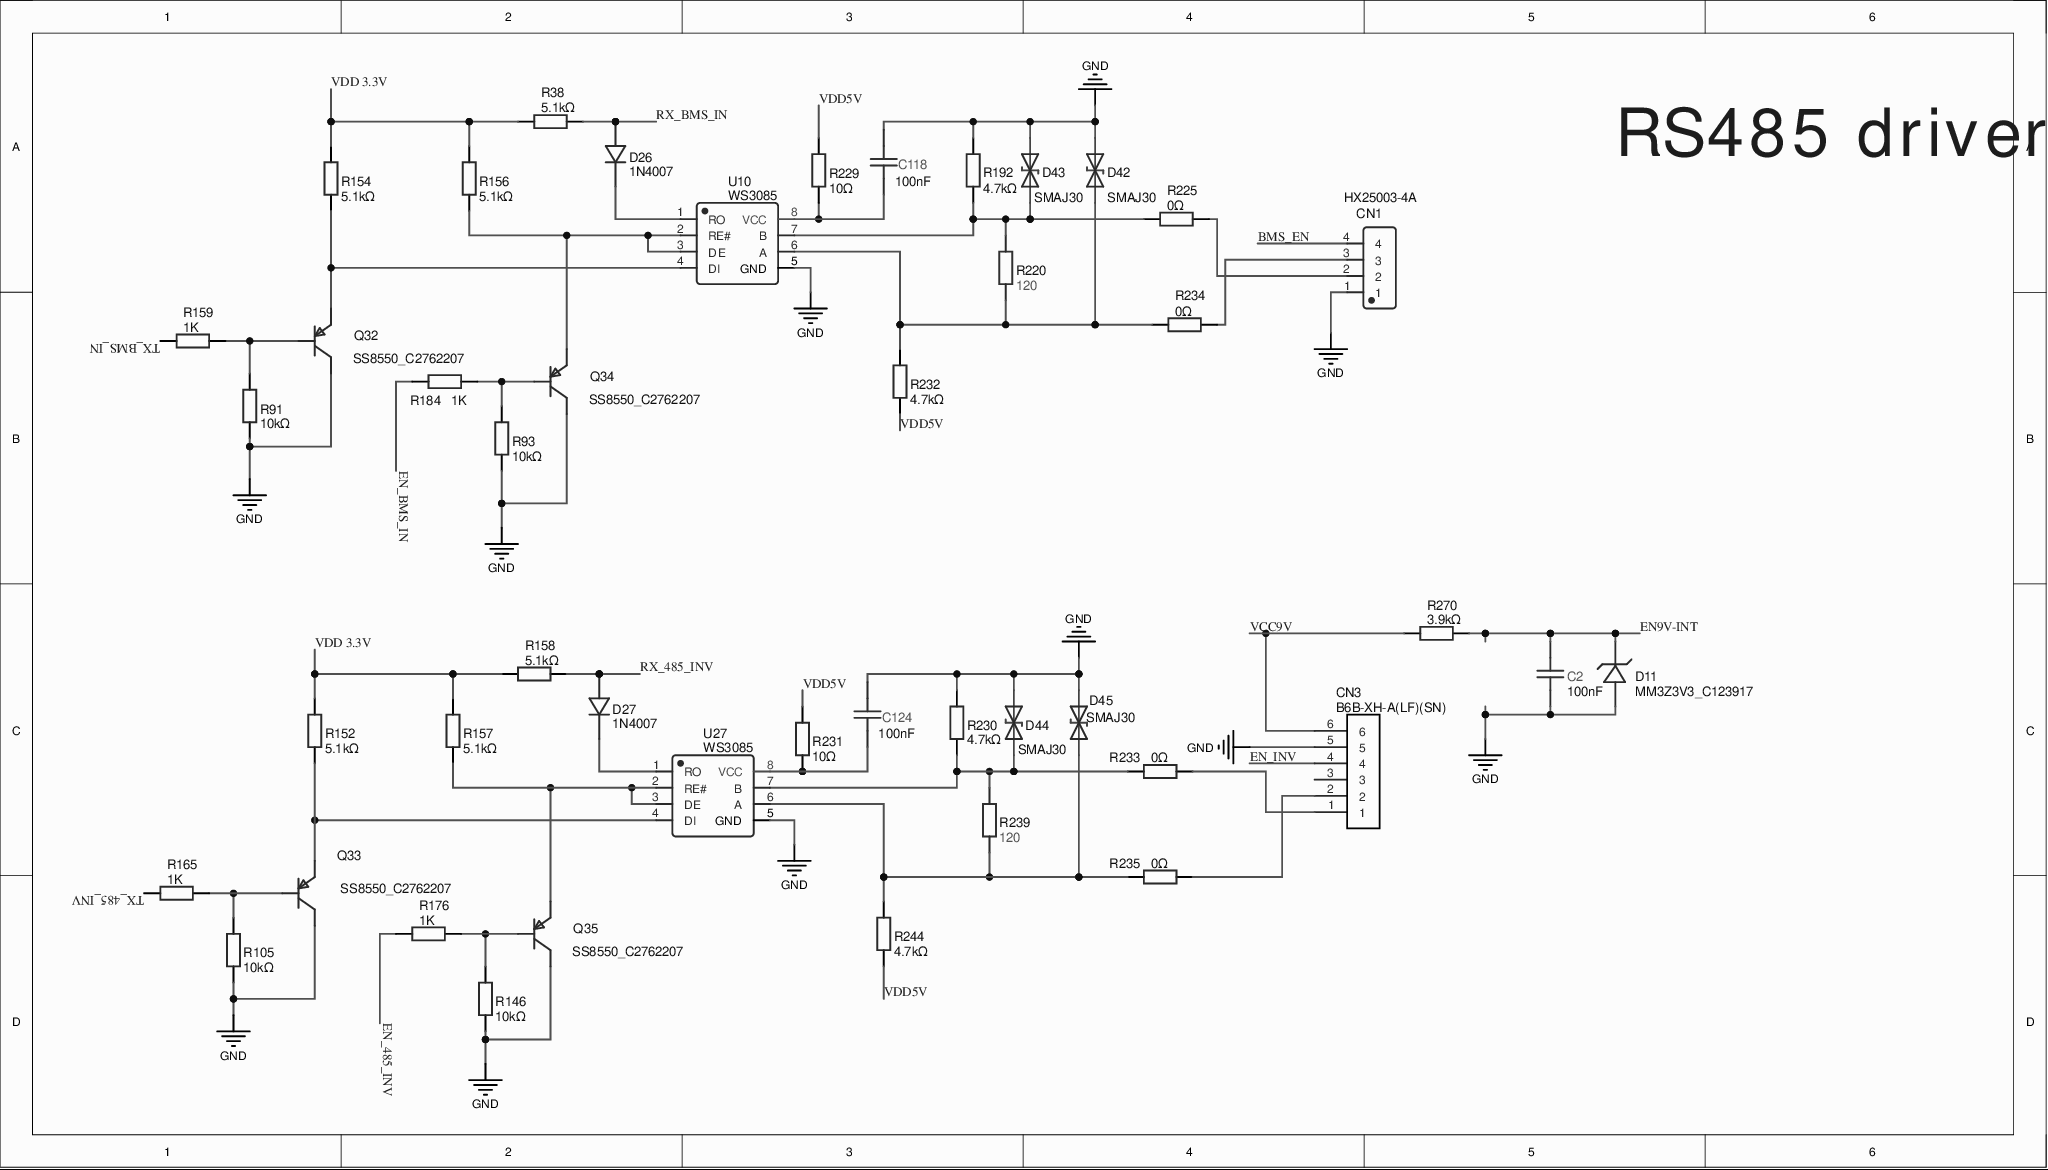
[diagram p0: MISC84402-10.SchDoc]
# Altium project MISC84402-4.PrjPcb (part 3 of 7)

## Sheet MISC84402-10.SchDoc
size 319 x 182 mm

### Parts
C2  100nF  [C0603]
C118  100nF  [C0603]
C124  100nF  [C0603]
CN1  HX25003-4A  [CONN-TH_4P-P2.50_HX25003-4A]
CN3  B6B-XH-A(LF)(SN)  [CONN-TH_6P-P2.50_B6B-XH-A-LF-SN]
D11  MM3Z3V3_C123917  [SOD-323_L1.8-W1.3-LS2.5-RD]
D26  1N4007  [DO-41_BD2.4-L4.7-P8.70-D0.9-RD]
D27  1N4007  [DO-41_BD2.4-L4.7-P8.70-D0.9-RD]
D42  SMAJ30  [SMA_L4.3-W2.5-LS5.0-BI]
D43  SMAJ30  [SMA_L4.3-W2.5-LS5.0-BI]
D44  SMAJ30  [SMA_L4.3-W2.5-LS5.0-BI]
D45  SMAJ30  [SMA_L4.3-W2.5-LS5.0-BI]
Q32  SS8550_C2762207  [SOT-23-3_L2.9-W1.3-P1.90-LS2.4-BR]
Q33  SS8550_C2762207  [SOT-23-3_L2.9-W1.3-P1.90-LS2.4-BR]
Q34  SS8550_C2762207  [SOT-23-3_L2.9-W1.3-P1.90-LS2.4-BR]
Q35  SS8550_C2762207  [SOT-23-3_L2.9-W1.3-P1.90-LS2.4-BR]
R38  5.1kΩ  [R0603]
R91  10kΩ  [R0603]
R93  10kΩ  [R0603]
R105  10kΩ  [R0603]
R146  10kΩ  [R0603]
R152  5.1kΩ  [R0603]
R154  5.1kΩ  [R0603]
R156  5.1kΩ  [R0603]
R157  5.1kΩ  [R0603]
R158  5.1kΩ  [R0603]
R159  1K  [R0603]
R165  1K  [R0603]
R176  1K  [R0603]
R184  1K  [R0603]
R192  4.7kΩ  [R0603]
R220  120  [R1206]
R225  0Ω  [R0603]
R229  10Ω  [R0603]
R230  4.7kΩ  [R0603]
R231  10Ω  [R0603]
R232  4.7kΩ  [R0603]
R233  0Ω  [R0603]
R234  0Ω  [R0603]
R235  0Ω  [R0603]
R239  120  [R1206]
R244  4.7kΩ  [R0603]
R270  3.9kΩ  [R0603]
U10  WS3085  [SOP-8_L5.0-W4.0-P1.27-LS6.0-BL]
U27  WS3085  [SOP-8_L5.0-W4.0-P1.27-LS6.0-BL]

### Nets
GND: C2.1 C118.2 C124.2 CN1.1 CN3.5 D11.2(A) D42.2 D43.2 D44.2 D45.2 Q32.3(C) Q33.3(C) Q34.3(C) Q35.3(C) R91.1 R93.1 R105.1 R146.1 R192.2 R230.2 U10.5(GND) U27.5(GND)
BMS_EN: CN1.4
EN9V-INT: C2.2 D11.1(K) R270.2
EN_485_INV: R176.1
EN_BMS_IN: R184.1
EN_INV: CN3.4
RX_485_INV: D27.2 R158.2
RX_BMS_IN: D26.2 R38.2
TX_485_INV: R165.1
TX_BMS_IN: R159.1
VCC9V: CN3.6 R270.1
VDD5V: R229.2 R231.2 R232.1 R244.1
VDD 3.3V: R38.1 R152.2 R154.2 R156.2 R157.2 R158.1
NetC118_1: C118.1 R229.1 U10.8(VCC)
NetC124_1: C124.1 R231.1 U27.8(VCC)
NetCN1_2: CN1.2 R225.2
NetCN1_3: CN1.3 R234.2
NetCN3_1: CN3.1 R233.2
NetCN3_2: CN3.2 R235.2
NetD26_1: D26.1 U10.1(RO)
NetD27_1: D27.1 U27.1(RO)
NetD42_1: D42.1 R220.1 R232.2 R234.1 U10.6(A)
NetD43_1: D43.1 R192.1 R220.2 R225.1 U10.7(B)
NetD44_1: D44.1 R230.1 R233.1 R239.1 U27.7(B)
NetD45_1: D45.1 R235.1 R239.2 R244.2 U27.6(A)
NetQ32_1: Q32.1(B) R91.2 R159.2
NetQ32_2: Q32.2(E) R154.1 U10.4(DI)
NetQ33_1: Q33.1(B) R105.2 R165.2
NetQ33_2: Q33.2(E) R152.1 U27.4(DI)
NetQ34_1: Q34.1(B) R93.2 R184.2
NetQ34_2: Q34.2(E) R156.1 U10.2(RE#) U10.3(DE)
NetQ35_1: Q35.1(B) R146.2 R176.2
NetQ35_2: Q35.2(E) R157.1 U27.2(RE#) U27.3(DE)

Not connected (* = marked no-connect by the designer): CN3 3

### Notes on the sheet
- RS485 driver circuit

### Library data of the parts
C2 C118 C124 = 100nF: BOM_Manufacturer: SAMSUNG; BOM_Manufacturer Part: CL10B104KC8NNNC; nameAlias: Capacitance; BOM_Supplier: LCSC; BOM_Supplier Part: C15725; BOM_JLCPCB Part Class: Extended Part; spicePre: C; spiceSymbolName: CL10B104KC8NNNC
CN1 = HX25003-4A: BOM_Manufacturer: HX(Zhejiang Yueqing Hongxing Elec); Contributor: LCSC; BOM_Supplier: LCSC; BOM_Supplier Part: C442301; BOM_Manufacturer Part: HX25003-4A; BOM_JLCPCB Part Class: Extended Part; spicePre: C; spiceSymbolName: HX25003-4A
CN3 = B6B-XH-A(LF)(SN): BOM_Manufacturer: JST Sales America; Contributor: LCSC; BOM_Supplier: LCSC; BOM_Supplier Part: C144397; BOM_Manufacturer Part: B6B-XH-A(LF)(SN); BOM_JLCPCB Part Class: Extended Part; spicePre: U; spiceSymbolName: B6B-XH-A(LF)(SN)
D11 = MM3Z3V3_C123917: BOM_Manufacturer: Shandong Jingdao Microelectronics; Contributor: LCSC; BOM_Supplier: LCSC; BOM_Supplier Part: C123917; BOM_Manufacturer Part: MM3Z3V3; BOM_JLCPCB Part Class: Extended Part; spicePre: D; spiceSymbolName: MM3Z3V3_C123917
D26 D27 = 1N4007: BOM_Manufacturer: SEMTECH; Contributor: LCEDA_Lib; BOM_Supplier: LCSC; BOM_Manufacturer Part: 1N4007; BOM_Supplier Part: C106903; spicePre: D; spiceSymbolName: 1N4007
D42-D45 = SMAJ30: BOM_Manufacturer: Shandong Jingdao Microelectronics; BOM_Manufacturer Part: SMAJ30CA; Contributor: LCSC; BOM_Supplier: LCSC; BOM_Supplier Part: C353455; BOM_JLCPCB Part Class: Extended Part; spicePre: D; spiceSymbolName: SMAJ30CA_C353455
Q32-Q35 = SS8550_C2762207: BOM_Manufacturer: Jingdao Microelectronics; BOM_Manufacturer Part: SS8550; Contributor: LCSC; BOM_Supplier: LCSC; BOM_Supplier Part: C2762207; BOM_JLCPCB Part Class: Extended Part; spicePre: Q; spiceSymbolName: SS8550_C2762207
R38 R152 R154 R156-R158 = 5.1kΩ: BOM_Manufacturer Part: 0603WAF5101T5E; BOM_Manufacturer: UniOhm; Resistance (Ohms): 5.1K; nameAlias: Resistance; BOM_Supplier: LCSC; BOM_Supplier Part: C23186; BOM_JLCPCB Part Class: Basic Part; spicePre: R; spiceSymbolName: 0603WAF5101T5E
R91 R93 R105 R146 = 10kΩ: BOM_Manufacturer: UniOhm; BOM_Manufacturer Part: 0603WAF1002T5E; nameAlias: Resistance; Resistance (Ohms): 10K; BOM_Supplier: LCSC; BOM_Supplier Part: C25804; BOM_JLCPCB Part Class: Basic Part; spicePre: R; spiceSymbolName: 0603WAF1002T5E
R159 R165 R176 R184 = 1K: BOM_Manufacturer: FH; BOM_Manufacturer Part: RS-03K102JT; nameAlias: Resistance (Ohms); BOM_Supplier: LCSC; BOM_Supplier Part: C73797; spicePre: R; spiceSymbolName: RS-03K102JT
R192 R230 R232 R244 = 4.7kΩ: BOM_Manufacturer: UniOhm; BOM_Manufacturer Part: 0603WAF4701T5E; nameAlias: Resistance; Resistance (Ohms): 4.7K; BOM_Supplier: LCSC; BOM_Supplier Part: C23162; BOM_JLCPCB Part Class: Basic Part; spicePre: R; spiceSymbolName: 0603WAF4701T5E
R220 R239 = 120: BOM_Manufacturer: Viking Tech; BOM_Manufacturer Part: ARG06FTC1200; nameAlias: Resistance (Ohms); Contributor: LCSC; BOM_Supplier: LCSC; BOM_Supplier Part: C294122; BOM_JLCPCB Part Class: Extended Part; spicePre: R; spiceSymbolName: ARG06FTC1200
R225 R233-R235 = 0Ω: BOM_Manufacturer: UniOhm; BOM_Manufacturer Part: 0603WAF0000T5E; nameAlias: Resistance; Resistance (Ohms): 0; BOM_Supplier: LCSC; BOM_Supplier Part: C21189; BOM_JLCPCB Part Class: Basic Part; spicePre: R; spiceSymbolName: 0603WAF0000T5E
R229 R231 = 10Ω: BOM_Manufacturer: UniOhm; BOM_Manufacturer Part: 0603WAF100JT5E; nameAlias: Resistance; BOM_Supplier: LCSC; BOM_Supplier Part: C22859; Resistance (Ohms): 10Ω; BOM_JLCPCB Part Class: Basic Part; spicePre: R; spiceSymbolName: 0603WAF100JT5E
R270 = 3.9kΩ: BOM_Manufacturer: UniOhm; BOM_Manufacturer Part: 0603WAF3901T5E; nameAlias: Resistance; Resistance (Ohms): 3.9K; BOM_Supplier: LCSC; BOM_Supplier Part: C23018; BOM_JLCPCB Part Class: Basic Part; spicePre: R; spiceSymbolName: 0603WAF3901T5E
U10 U27 = WS3085: BOM_Manufacturer: GEC (Nanjing Guobo); Contributor: LCSC; BOM_Supplier: LCSC; BOM_Supplier Part: C2691412; BOM_Manufacturer Part: WS3085; BOM_JLCPCB Part Class: Extended Part; spicePre: U; spiceSymbolName: WS3085

## Sheet MISC84402-9.SchDoc
size 225 x 98 mm
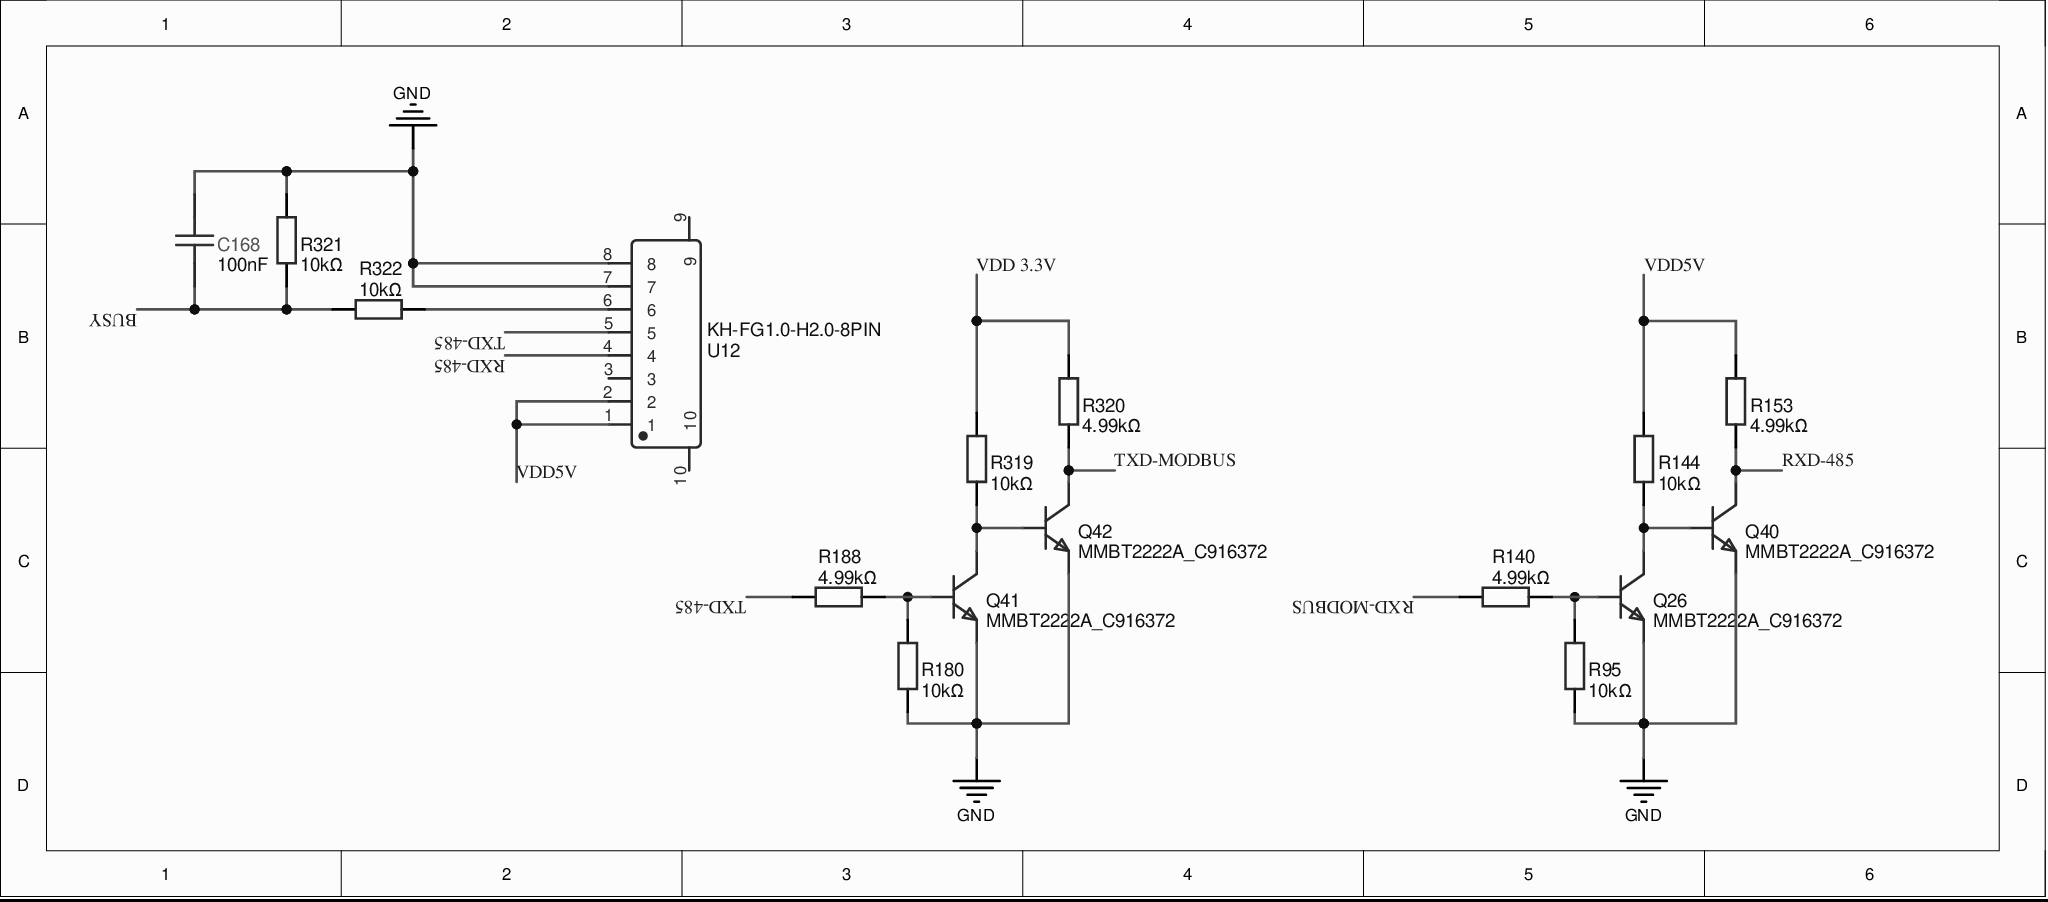
[diagram p1: MISC84402-9.SchDoc]

### Parts
C168  100nF  [C0603]
Q26  MMBT2222A_C916372  [SOT-23-3_L2.9-W1.3-P1.90-LS2.4-BR]
Q40  MMBT2222A_C916372  [SOT-23-3_L2.9-W1.3-P1.90-LS2.4-BR]
Q41  MMBT2222A_C916372  [SOT-23-3_L2.9-W1.3-P1.90-LS2.4-BR]
Q42  MMBT2222A_C916372  [SOT-23-3_L2.9-W1.3-P1.90-LS2.4-BR]
R95  10kΩ  [R0603]
R140  4.99kΩ  [R0603]
R144  10kΩ  [R0603]
R153  4.99kΩ  [R0603]
R180  10kΩ  [R0603]
R188  4.99kΩ  [R0603]
R319  10kΩ  [R0603]
R320  4.99kΩ  [R0603]
R321  10kΩ  [R0603]
R322  10kΩ  [R0603]
U12  KH-FG1.0-H2.0-8PIN  [FPC-SMD_KH-FG1.0-H2.0-8PIN]

### Nets
GND: C168.1 Q26.2(E) Q40.2(E) Q41.2(E) Q42.2(E) R95.1 R180.1 R321.2 U12.7 U12.8
BUSY: C168.2 R321.1 R322.2
RXD-485: Q40.3(C) R153.1 U12.4
RXD-MODBUS: R140.1
TXD-485: R188.2 U12.5
TXD-MODBUS: Q42.3(C) R320.1
VDD5V: R144.2 R153.2 U12.1 U12.2
VDD 3.3V: R319.2 R320.2
NetQ26_1: Q26.1(B) R95.2 R140.2
NetQ26_3: Q26.3(C) Q40.1(B) R144.1
NetQ41_1: Q41.1(B) R180.2 R188.1
NetQ41_3: Q41.3(C) Q42.1(B) R319.1
NetR322_1: R322.1 U12.6

Not connected (* = marked no-connect by the designer): U12 3 9 10

### Library data of the parts
C168 = 100nF: as C2 on sheet MISC84402-10; BOM_Supplier: LCSC; BOM_Supplier Part: C15725; BOM_JLCPCB Part Class: Extended Part; spicePre: C; spiceSymbolName: CL10B104KC8NNNC
Q26 Q40-Q42 = MMBT2222A_C916372: BOM_Manufacturer: JSMSEMI; Contributor: LCSC; BOM_Supplier: LCSC; BOM_Supplier Part: C916372; BOM_Manufacturer Part: MMBT2222A; BOM_JLCPCB Part Class: Extended Part; spicePre: Q; spiceSymbolName: MMBT2222A_C916372
R95 R144 R180 R319 R321 R322 = 10kΩ: as R91 on sheet MISC84402-10; BOM_Supplier: LCSC; BOM_Supplier Part: C25804; BOM_JLCPCB Part Class: Basic Part; spicePre: R; spiceSymbolName: 0603WAF1002T5E
R140 R153 R188 R320 = 4.99kΩ: BOM_Manufacturer: UniOhm; BOM_Manufacturer Part: 0603WAF4991T5E; nameAlias: Resistance; Resistance (Ohms): 4.99K; BOM_Supplier: LCSC; BOM_Supplier Part: C23046; BOM_JLCPCB Part Class: Basic Part; spicePre: R; spiceSymbolName: 0603WAF4991T5E
U12 = KH-FG1.0-H2.0-8PIN: BOM_Manufacturer: Kinghelm; Contributor: LCSC; BOM_Supplier: LCSC; BOM_Supplier Part: C2797225; BOM_Manufacturer Part: KH-FG1.0-H2.0-8PIN; BOM_JLCPCB Part Class: Extended Part; spicePre: C; spiceSymbolName: KH-FG1.0-H2.0-8PIN

## Sheet MISC84402-11.SchDoc
size 345 x 185 mm
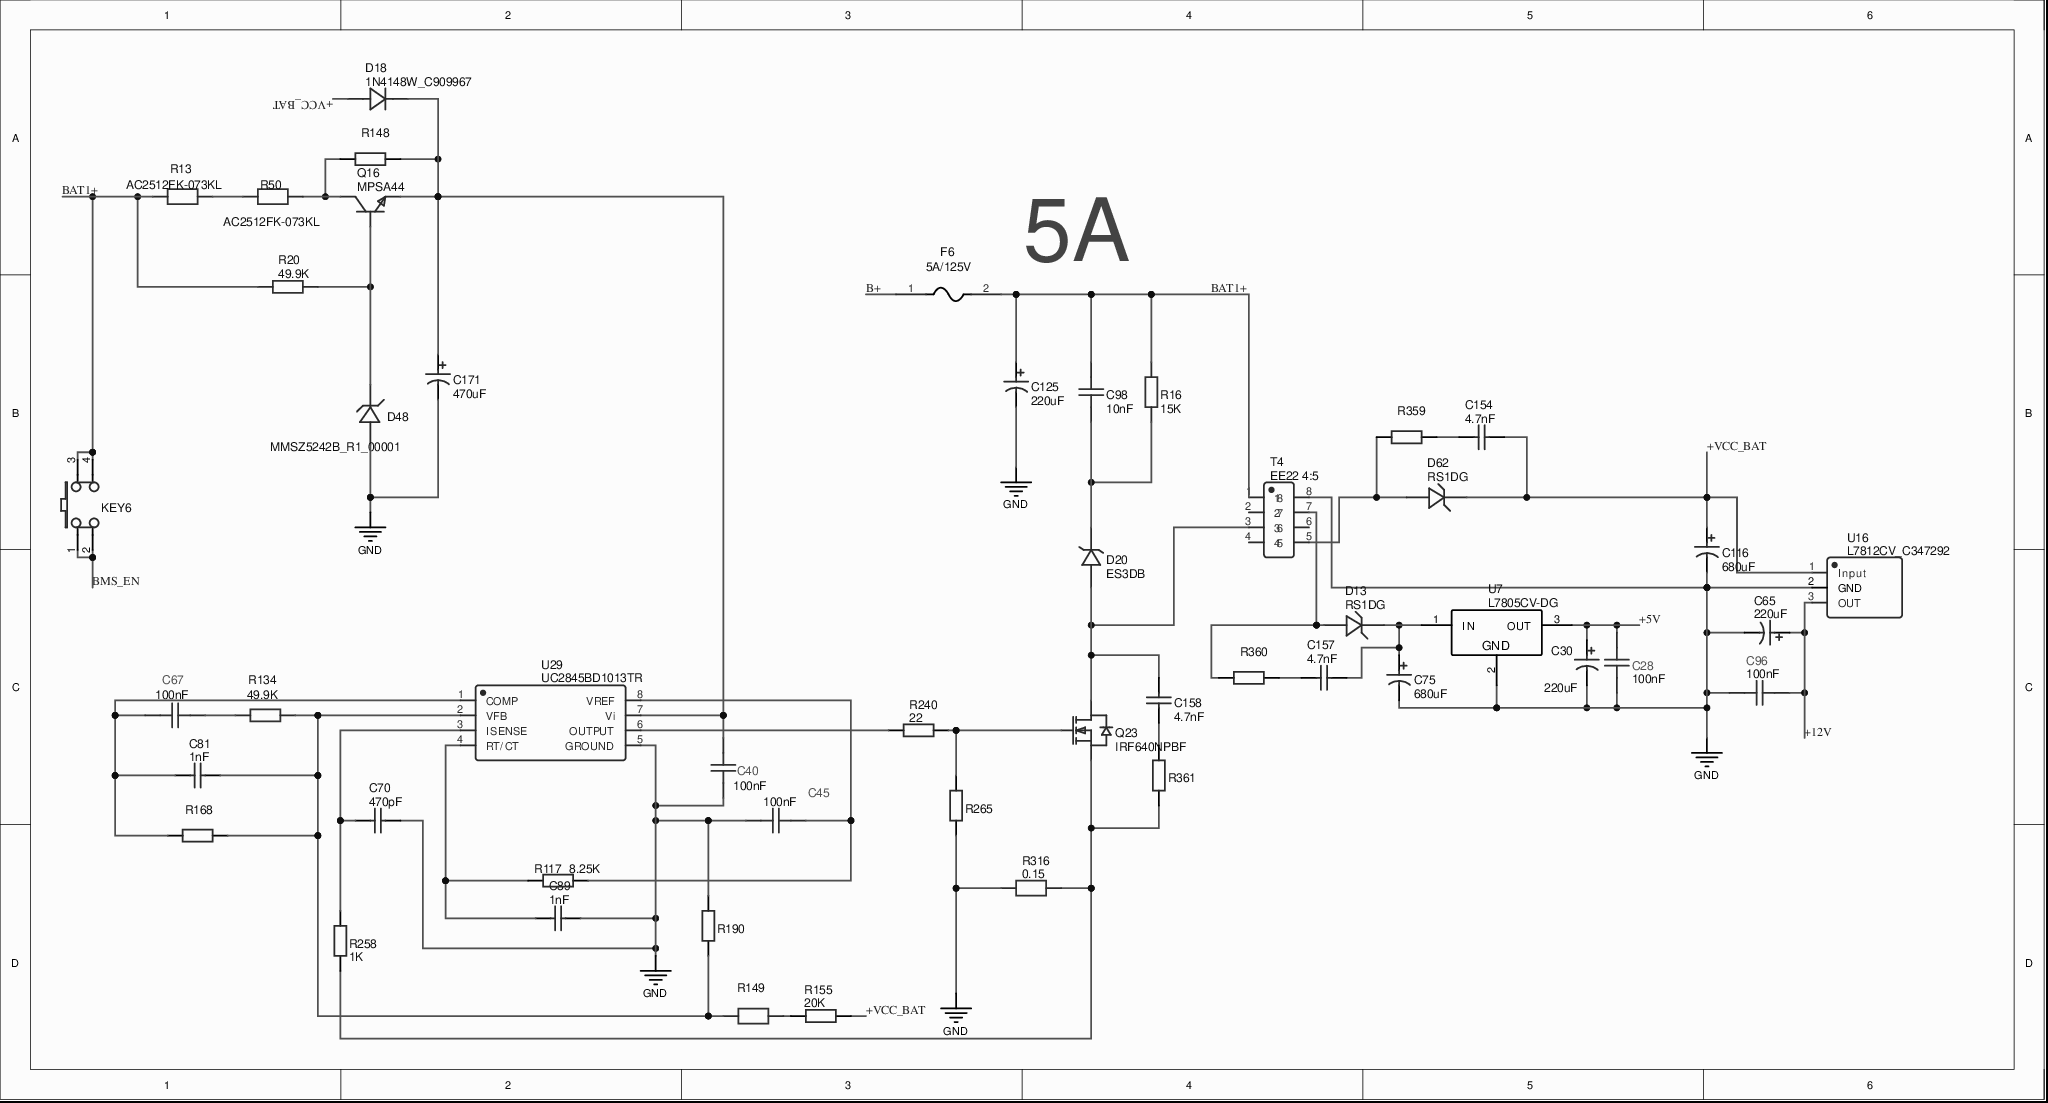
[diagram p2: MISC84402-11.SchDoc]

### Parts
C28  100nF  [C0603]
C30  220uF  [CAP-TH_BD6.3-P2.50-D1.0-FD]
C40  100nF  [C0603]
C45  100nF  [C0603]
C65  220uF  [CAP-TH_BD6.3-P2.50-D1.0-FD]
C67  100nF  [C0603]
C70  470pF  [C0603]
C75  680uF  [CAP-TH_BD10.0-P5.00-D1.0-FD]
C81  1nF  [C0603]
C89  1nF  [C0603]
C96  100nF  [C0603]
C98  10nF  [CAP-TH_L8.0-W4.0-P5.00-D1.2]
C116  680uF  [CAP-TH_BD10.0-P5.00-D1.0-FD]
C125  220uF  [CAP-TH_BD10.0-P5.00-D1.0-FD]
C154  4.7nF  [C1206]
C157  4.7nF  [C1206]
C158  4.7nF  [C1206]
C171  470uF  [CAP-TH_BD12.5-P5.00-D0.6-FD]
D13  RS1DG  [SMA_L4.4-W2.8-LS5.4-RD]
D18  1N4148W_C909967  [SOD-123_L2.8-W1.8-LS3.7-RD]
D20  ES3DB  [SMB_L4.6-W3.6-LS5.3-RD]
D48  MMSZ5242B_R1_00001  [SOD-123_L2.7-W1.6-LS3.7-RD-1]
D62  RS1DG  [SMA_L4.4-W2.8-LS5.4-RD]
F6  5A/125V  [FUSE-SMD_L6.1-W2.5]
KEY6  4-1437565-2  [SW-SMD_4P-L6.0-W6.0-P4.50-LS8.6]  (value not drawn)
Q16  MPSA44  [TO-92-3_L4.8-W3.7-P2.54-L]
Q23  IRF640NPBF  [TO-220-3_L10.0-W4.5-P2.54-L]
R13  AC2512FK-073KL  [R2512]
R16  15K  [RES-TH_BD3.3-L9.0-P13.00-D0.6]
R20  49.9K  [R0603]
R50  AC2512FK-073KL  [R2512]
R117  8.25K  [R0603]
R134  49.9K  [R0603]
R148  (no value)  [R0603]
R149  (no value)  [R0603]
R155  20K  [R0603]
R168  (no value)  [R0603]
R190  (no value)  [R0603]
R240  22  [R0603]
R258  1K  [R0603]
R265  (no value)  [R0603]
R316  0.15  [R2512]
R359  (no value)  [R1206]
R360  (no value)  [R1206]
R361  (no value)  [R1206]
T4  EE22 4:5  [EE22 4:5NEW]
U7  L7805CV-DG  [TO-220-3_L10.0-W4.5-P2.54-L]
U16  L7812CV_C347292  [TO-220-3_L10.0-W4.5-P2.54-L]
U29  UC2845BD1013TR  [SOP-8_L4.9-W3.9-P1.27-LS6.0-BL]

### Nets
GND: C28.2 C30.2 C40.1 C45.2 C65.2 C70.2 C75.2 C89.2 C96.2 C116.2 C125.2 C171.2 D48.2(A) R190.2 R265.1 R316.1 T4.8 U7.2(GND) U16.2(GND) U29.5(GROUND)
+5V: C28.1 C30.1 U7.3(OUT)
+12V: C65.1 C96.1 U16.3(OUT)
+VCC_BAT: C116.1 C154.1 D18.2(A) D62.1(C) R155.1 U16.1(Input)
B+: F6.1
BAT1+: C98.2 C125.1 F6.2 KEY6.3 KEY6.4 R13.2 R16.2 R20.1 T4.1
BMS_EN: KEY6.1 KEY6.2
NetC40_2: C40.2 C171.1 D18.1(K) Q16.1(E) R148.2 U29.7(Vi)
NetC45_1: C45.1 R117.2 U29.8(VREF)
NetC67_1: C67.1 R134.1
NetC67_2: C67.2 C81.1 R168.2 U29.1(COMP)
NetC70_1: C70.1 R258.2 U29.3(ISENSE)
NetC75_1: C75.1 C157.1 D13.1(C) U7.1(IN)
NetC81_2: C81.2 R134.2 R149.2 R168.1 R190.1 U29.2(VFB)
NetC89_1: C89.1 R117.1 U29.4(RT/CT)
NetC98_1: C98.1 D20.1(C) R16.1
NetC154_2: C154.2 R359.2
NetC157_2: C157.2 R360.2
NetC158_1: C158.1 R361.2
NetC158_2: C158.2 D20.2(A) Q23.2(D) T4.3
NetD13_2: D13.2(A) R360.1 T4.7
NetD48_1: D48.1(K) Q16.2(B) R20.2
NetD62_2: D62.2(A) R359.1 T4.5
NetQ16_3: Q16.3(C) R50.1 R148.1
NetQ23_1: Q23.1(G) R240.2 R265.2
NetQ23_3: Q23.3(S) R258.1 R316.2 R361.1
NetR13_1: R13.1 R50.2
NetR149_1: R149.1 R155.2
NetR240_1: R240.1 U29.6(OUTPUT)

Not connected (* = marked no-connect by the designer): T4 2 4 6

### Notes on the sheet
- (near F6) 5A

### Library data of the parts
C28 C40 C45 C67 C96 = 100nF: as C2 on sheet MISC84402-10; BOM_Supplier: LCSC; BOM_Supplier Part: C15725; BOM_JLCPCB Part Class: Extended Part; spicePre: C; spiceSymbolName: CL10B104KC8NNNC
C30 C65 = 220uF: BOM_Manufacturer: ValuePro; BOM_Manufacturer Part: 220uF 16V 6.3*11; nameAlias: Capacitance; BOM_Supplier: LCSC; BOM_Supplier Part: C43349; BOM_JLCPCB Part Class: Extended Part; spicePre: C; spiceSymbolName: 220uF 16V 6.3*11
C70 = 470pF: BOM_Manufacturer: FH; BOM_Manufacturer Part: 0603B471K500NT; nameAlias: Capacitance; BOM_Supplier: LCSC; BOM_Supplier Part: C1620; BOM_JLCPCB Part Class: Basic Part; spicePre: C; spiceSymbolName: 0603B471K500NT
C75 C116 = 680uF: BOM_Manufacturer: ValuePro; BOM_Manufacturer Part: high frequency 680uF35V; nameAlias: Capacitance; BOM_Supplier: LCSC; BOM_Supplier Part: C23777; BOM_JLCPCB Part Class: Extended Part; spicePre: C; spiceSymbolName: high frequency 680uF35V
C81 C89 = 1nF: BOM_Manufacturer Part: CL10B102KB8NNNC; BOM_Manufacturer: SAMSUNG; nameAlias: Capacitance; BOM_Supplier: LCSC; BOM_Supplier Part: C1588; BOM_JLCPCB Part Class: Basic Part; spicePre: C; spiceSymbolName: CL10B102KB8NNNC
C98 = 10nF: BOM_Manufacturer: Songtian Elec; BOM_Manufacturer Part: N09F1B103MN0B0S0N0; nameAlias: Capacitance; Contributor: LCSC; BOM_Supplier: LCSC; BOM_Supplier Part: C249157; BOM_JLCPCB Part Class: Extended Part; spicePre: C; spiceSymbolName: N09F1B103MN0B0S0N0
C125 = 220uF: BOM_Manufacturer: ValuePro; BOM_Manufacturer Part: 220uf/63V; nameAlias: Capacitance; BOM_Supplier: LCSC; BOM_Supplier Part: C47290; BOM_JLCPCB Part Class: Extended Part; spicePre: C; spiceSymbolName: 220uf/63V
C154 C157 C158 = 4.7nF: BOM_Manufacturer: FH; BOM_Manufacturer Part: 1206B472K102NT; nameAlias: Capacitance; BOM_Supplier: LCSC; BOM_Supplier Part: C9192; BOM_JLCPCB Part Class: Extended Part; spicePre: C; spiceSymbolName: 1206B472K102NT
C171 = 470uF: BOM_Manufacturer: ValuePro; nameAlias: Capacitance; BOM_Supplier: LCSC; BOM_Supplier Part: C18823; BOM_JLCPCB Part Class: Extended Part; spicePre: C
D13 D62 = RS1DG: Contributor: LCSC; BOM_Supplier: LCSC; BOM_Supplier Part: C472689; BOM_Manufacturer Part: RS1DG; BOM_JLCPCB Part Class: Extended Part; spicePre: D; spiceSymbolName: RS1DG
D18 = 1N4148W_C909967: BOM_Manufacturer: GOODWORK; Contributor: LCSC; BOM_Supplier: LCSC; BOM_Supplier Part: C909967; BOM_Manufacturer Part: 1N4148W; BOM_JLCPCB Part Class: Extended Part; spicePre: D; spiceSymbolName: 1N4148W_C909967
D20 = ES3DB: BOM_Manufacturer: Shandong Jingdao Microelectronics; Contributor: LCSC; BOM_Supplier: LCSC; BOM_Supplier Part: C437854; BOM_Manufacturer Part: ES3DB; BOM_JLCPCB Part Class: Extended Part; spicePre: D; spiceSymbolName: ES3DB
D48 = MMSZ5242B_R1_00001: BOM_Manufacturer: PANJIT International; Contributor: LCSC; BOM_Supplier: LCSC; BOM_Supplier Part: C268606; BOM_Manufacturer Part: MMSZ5242B_R1_00001; BOM_JLCPCB Part Class: Extended Part; spicePre: D; spiceSymbolName: MMSZ5242B_R1_00001
F6 = 5A/125V: BOM_Manufacturer: RUILON; BOM_Supplier: LCSC; BOM_Supplier Part: C30198; BOM_JLCPCB Part Class: Extended Part; spicePre: F
KEY6 = 4-1437565-2: BOM_Manufacturer: TE Connectivity; BOM_Supplier: LCSC; BOM_Manufacturer Part: 4-1437565-2; BOM_Supplier Part: C86487; BOM_JLCPCB Part Class: Extended Part; spicePre: K; spiceSymbolName: 4-1437565-2
Q16 = MPSA44: BOM_Manufacturer: SEMTECH; Contributor: LCSC; BOM_Supplier: LCSC; BOM_Manufacturer Part: MPSA44; BOM_Supplier Part: C157665; BOM_JLCPCB Part Class: Extended Part; spicePre: Q; spiceSymbolName: MPSA44
Q23 = IRF640NPBF: BOM_Manufacturer: Infineon; BOM_Supplier: LCSC; BOM_Manufacturer Part: IRF640NPBF; BOM_Supplier Part: C2568; BOM_JLCPCB Part Class: Extended Part; spicePre: Q; spiceSymbolName: IRF640NPBF
R13 R50 = AC2512FK-073KL: BOM_Manufacturer: YAGEO; Contributor: LCSC; BOM_Supplier: LCSC; BOM_Supplier Part: C728188; BOM_Manufacturer Part: AC2512FK-073KL; BOM_JLCPCB Part Class: Extended Part; spicePre: R; spiceSymbolName: AC2512FK-073KL
R16 = 15K: BOM_Manufacturer: TyoHM; nameAlias: Resistance (Ohms); Contributor: LCSC; BOM_Supplier: LCSC; BOM_Supplier Part: C385283; BOM_JLCPCB Part Class: Extended Part; spicePre: R
R20 R134 = 49.9K: BOM_Manufacturer: Tyohm; BOM_Manufacturer Part: RMC060349.9K1%N; nameAlias: Resistance (Ohms); Contributor: LCSC; BOM_Supplier: LCSC; BOM_Supplier Part: C325621; spicePre: R; spiceSymbolName: RMC060349.9K1%N
R117 = 8.25K: BOM_Manufacturer: UniOhm; BOM_Manufacturer Part: 0603WAF8251T5E; nameAlias: Resistance (Ohms); BOM_Supplier: LCSC; BOM_Supplier Part: C23113; BOM_JLCPCB Part Class: Extended Part; spicePre: R; spiceSymbolName: 0603WAF8251T5E
R148 = (no symbol name): BOM_Manufacturer: UniOhm; BOM_Manufacturer Part: 0603WAF2003T5E; nameAlias: Resistance; Resistance (Ohms): 200K; BOM_Supplier: LCSC; BOM_Supplier Part: C25811; BOM_JLCPCB Part Class: Basic Part; spicePre: R; spiceSymbolName: 0603WAF2003T5E
R149 = (no symbol name): BOM_Manufacturer Part: SY0603DD30KP; nameAlias: Resistance; Contributor: LCSC; BOM_Supplier: LCSC; BOM_Supplier Part: C2763744; BOM_JLCPCB Part Class: Extended Part; spicePre: R; spiceSymbolName: SY0603DD30KP
R155 = 20K: BOM_Manufacturer: YAGEO; BOM_Manufacturer Part: RC0603FR-0720KL; nameAlias: Resistance (Ohms); BOM_Supplier: LCSC; BOM_Supplier Part: C105575; BOM_JLCPCB Part Class: Extended Part; spicePre: R; spiceSymbolName: RC0603FR-0720KL
R168 = (no symbol name): BOM_Manufacturer: UniOhm; BOM_Manufacturer Part: 0603WAF1003T5E; nameAlias: Resistance; Resistance (Ohms): 100K; BOM_Supplier: LCSC; BOM_Supplier Part: C25803; BOM_JLCPCB Part Class: Basic Part; spicePre: R; spiceSymbolName: 0603WAF1003T5E
R190 = (no symbol name): BOM_Manufacturer: UniOhm; BOM_Manufacturer Part: 0603WAF1002T5E; nameAlias: Resistance; Resistance (Ohms): 10K; BOM_Supplier: LCSC; BOM_Supplier Part: C25804; BOM_JLCPCB Part Class: Basic Part; spicePre: R; spiceSymbolName: 0603WAF1002T5E
R240 = 22: BOM_Manufacturer: UniOhm; BOM_Manufacturer Part: 0603WAJ0220T5E; nameAlias: Resistance (Ohms); BOM_Supplier: LCSC; BOM_Supplier Part: C1203; BOM_JLCPCB Part Class: Extended Part; spicePre: R; spiceSymbolName: 0603WAJ0220T5E
R258 = 1K: as R159 on sheet MISC84402-10; BOM_Supplier: LCSC; BOM_Supplier Part: C73797; spicePre: R; spiceSymbolName: RS-03K102JT
R265 = (no symbol name): BOM_Manufacturer: UniOhm; BOM_Manufacturer Part: 0603WAF4702T5E; nameAlias: Resistance; Resistance (Ohms): 47K; BOM_Supplier: LCSC; BOM_Supplier Part: C25819; BOM_JLCPCB Part Class: Basic Part; spicePre: R; spiceSymbolName: 0603WAF4702T5E
R316 = 0.15: BOM_Manufacturer: SANYEAR; BOM_Manufacturer Part: SY2512CJR150; nameAlias: Resistance (Ohms); Contributor: LCSC; BOM_Supplier: LCSC; BOM_Supplier Part: C466831; BOM_JLCPCB Part Class: Extended Part; spicePre: R; spiceSymbolName: SY2512CJR150
R359-R361 = (no symbol name): BOM_Manufacturer: UniOhm; BOM_Manufacturer Part: 1206W4F220KT5E; nameAlias: Resistance; Resistance (Ohms): 2.2; BOM_Supplier: LCSC; BOM_Supplier Part: C17947; BOM_JLCPCB Part Class: Extended Part; spicePre: R; spiceSymbolName: 1206W4F220KT5E
T4 = EE22 4:5: BOM_Manufacturer: null; BOM_Manufacturer Part: EFD20_4X2F; Contributor: LCSC; BOM_Supplier: LCSC; BOM_Supplier Part: C2858319; BOM_JLCPCB Part Class: Extended Part; spicePre: U; spiceSymbolName: EFD20_4X2F
U7 = L7805CV-DG: BOM_Manufacturer: STMicroelectronics; BOM_Supplier: LCSC; BOM_Manufacturer Part: L7805CV-DG; BOM_Supplier Part: C3795; BOM_JLCPCB Part Class: Extended Part; spicePre: U; spiceSymbolName: L7805CV-DG
U16 = L7812CV_C347292: BOM_Manufacturer: Youtai Semiconductor Co., Ltd.; Contributor: LCSC; BOM_Supplier: LCSC; BOM_Supplier Part: C347292; BOM_Manufacturer Part: L7812CV; BOM_JLCPCB Part Class: Extended Part; spicePre: U; spiceSymbolName: L7812CV_C347292
U29 = UC2845BD1013TR: BOM_Manufacturer: STMicroelectronics; Contributor: LCSC; BOM_Supplier: LCSC; BOM_Supplier Part: C111203; BOM_Manufacturer Part: UC2845BD1013TR; BOM_JLCPCB Part Class: Extended Part; spicePre: U; spiceSymbolName: UC2845BD1013TR